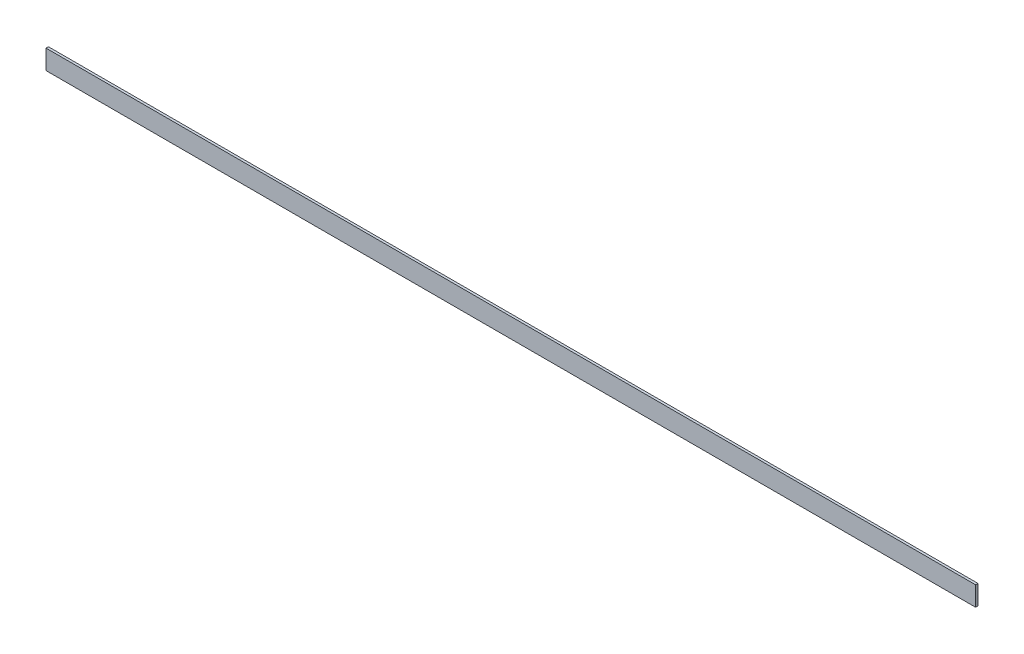
from build123d import *

# Parameters (mm, degrees)
SKETCH1_W           = 3100
SKETCH1_H           = 65
BOSS_EXTRUDE1_DEPTH = 8


with BuildPart() as part:
    # Sketch1 → Boss-Extrude1 (new body)
    with BuildSketch(Plane.XY):
        Rectangle(SKETCH1_W, SKETCH1_H)
    extrude(amount=BOSS_EXTRUDE1_DEPTH)


solid = part.part
